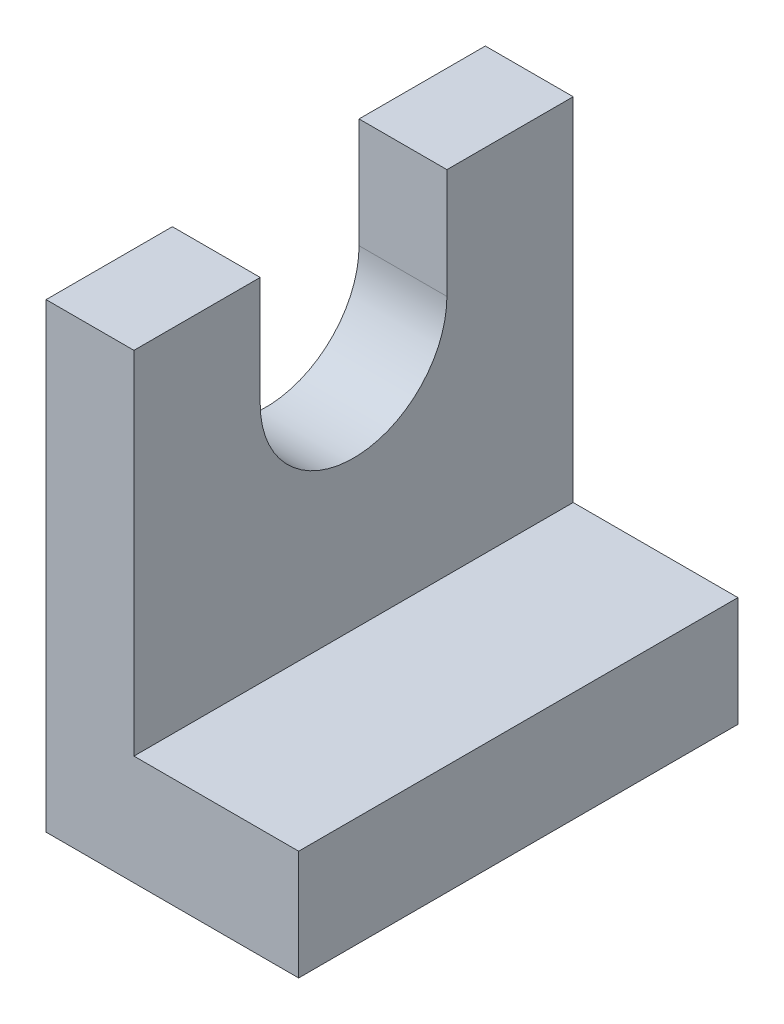
SolidWorks part; units mm, degrees
ref_plane "前视基准面" through (0, 0, 0) normal (0, 0, 1) x (1, 0, 0)
ref_plane "上视基准面" through (0, 0, 0) normal (0, 1, 0) x (1, 0, 0)
ref_plane "右视基准面" through (0, 0, 0) normal (1, 0, 0) x (0, 0, -1)
sketch "草图1" plane through (0, 0, 0) normal (0, 0, 1) x (1, 0, 0)
  line L0 (0, 0) -> (23, 0)
  line L1 (23, 0) -> (23, 10)
  line L2 (23, 10) -> (8, 10)
  line L3 (8, 10) -> (8, 42)
  line L4 (8, 42) -> (0, 42)
  line L5 (0, 42) -> (0, 0)
  dimension "D1" = 8
  dimension "D2" = 32
  dimension "D3" = 10
  dimension "D4" = 15
extrude "凸台-拉伸1" add sketch "草图1" along normal mid plane 40
sketch "草图2" plane through (8, 0, 0) normal (1, 0, 0) x (0, 0, -1)
  line L0 (-8.5, 42) -> (-8.5, 32)
  line L1 (-20, 42) -> (20, 42) construction
  line L2 (8.5, 32) -> (8.5, 42)
  line L3 (8.5, 42) -> (-8.5, 42)
  arc A0 (-8.5, 32) -> (8.5, 32) centre (0, 32) ccw
  dimension "D1" = 8.5
  dimension "D2" = 10
extrude "切除-拉伸1" cut sketch "草图2" against normal up to next
